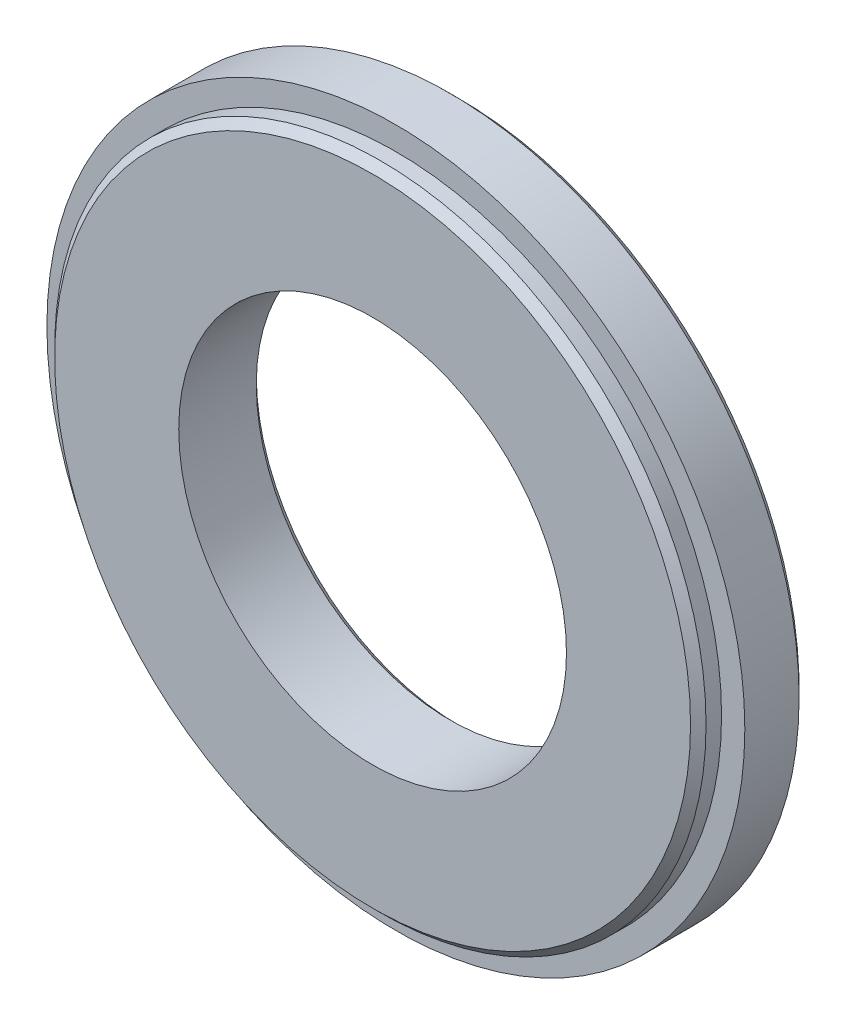
from build123d import *

# Parameters (mm, degrees)
SKETCH2_R             = 1.5
CUT_EXTRUDE1_DEPTH    = 3
M4_TAPPED_HOLE1_D     = 3.3
M4_TAPPED_HOLE1_DEPTH = 8
M4_TAPPED_HOLE1_TIP   = 0.991420021
CHAMFER1_SIZE         = 0.375
CHAMFER2_SIZE         = 1


with BuildPart() as part:
    # Sketch1 → Revolve1 (revolve)
    with BuildSketch(Plane(origin=(0, 0, 0), x_dir=(1, 0, 0), z_dir=(0, 1, 0))):
        Polygon((25, 0), (42, 0), (42, 3), (45, 3), (45, 11), (25, 11), align=None)
    revolve(axis=Axis((0, 0, 0), (0, 0, -1)))

    # Sketch2 → Cut-Extrude1 (cut)
    with BuildSketch(Plane(origin=(0, 0, -11), x_dir=(-1, 0, 0), z_dir=(0, 0, -1))):
        with Locations((0, -37)):
            Circle(SKETCH2_R)
        with Locations((-32.04293994, -18.5)):
            Circle(SKETCH2_R)
        with Locations((-32.04293994, 18.5)):
            Circle(SKETCH2_R)
        with Locations((0, 37)):
            Circle(SKETCH2_R)
        with Locations((32.04293994, 18.5)):
            Circle(SKETCH2_R)
        with Locations((32.04293994, -18.5)):
            Circle(SKETCH2_R)
    extrude(amount=-CUT_EXTRUDE1_DEPTH, mode=Mode.SUBTRACT)

    # M4 Tapped Hole1
    with Locations(Plane(origin=(0, 0, -11), x_dir=(-1, 0, 0), z_dir=(0, 0, -1))):
        with Locations((0, -37), (-32.04293994, -18.5), (-32.04293994, 18.5), (0, 37), (32.04293994, -18.5), (32.04293994, 18.5)):
            Hole(M4_TAPPED_HOLE1_D / 2, depth=M4_TAPPED_HOLE1_DEPTH)
            with Locations((0, 0, -(M4_TAPPED_HOLE1_DEPTH + M4_TAPPED_HOLE1_TIP / 2))):  # 118° drill point
                Cone(0, M4_TAPPED_HOLE1_D / 2, M4_TAPPED_HOLE1_TIP, mode=Mode.SUBTRACT)

    # Chamfer1
    chamfer1_edges = [part.edges().sort_by_distance(p)[0] for p in [
        (-33.69293994, 18.5, -11),
        (-33.69293994, -18.5, -11),
        (-1.65, 37, -11),
        (30.39293994, 18.5, -11),
        (30.39293994, -18.5, -11),
        (-1.65, -37, -11),
    ]]
    chamfer(chamfer1_edges, length=CHAMFER1_SIZE)

    # Chamfer2
    chamfer2_edges = [part.edges().sort_by_distance(p)[0] for p in [
        (-25, 0, -11),
        (-45, 0, -11),
        (-42, 0, 0),
    ]]
    chamfer(chamfer2_edges, length=CHAMFER2_SIZE)


solid = part.part
